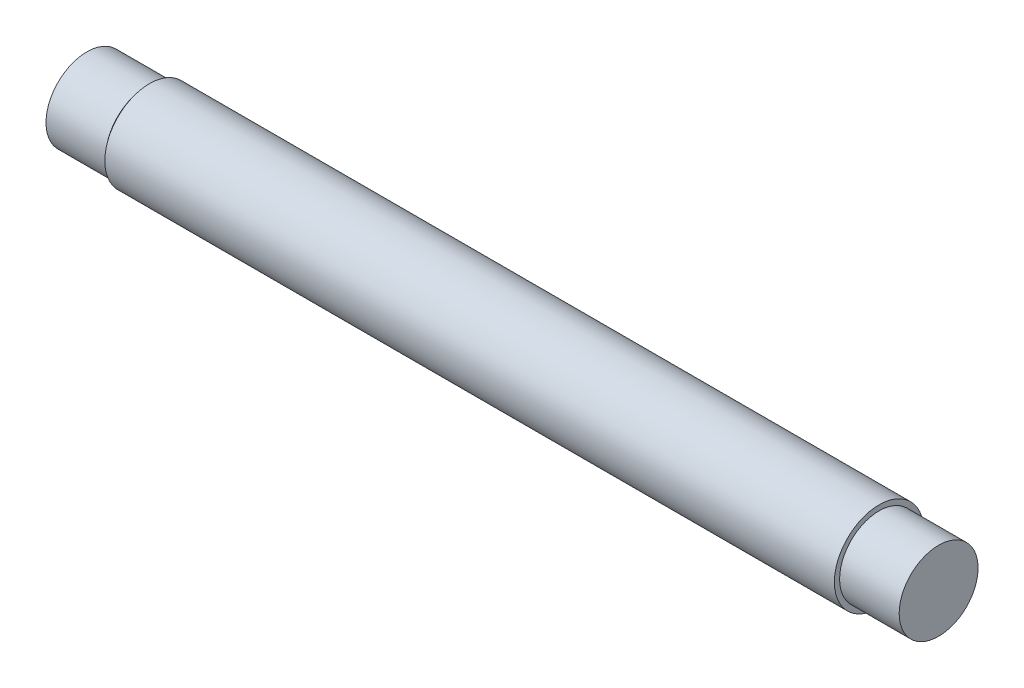
from build123d import *


with BuildPart() as part:
    # 草图1 → 旋转1 (revolve)
    with BuildSketch(Plane.XY, mode=Mode.PRIVATE) as revolve_1_sk:
        Polygon((0, 0), (0, 27.5), (40, 27.5), (40, 26.5), (42, 26.5), (42, 30), (532, 30), (532, 26.5), (572, 26.5), (572, 0), align=None)
    revolve(revolve_1_sk.sketch.rotate(Axis((0, 0, 0), (1, 0, 0)), 90), axis=Axis((0, 0, 0), (1, 0, 0)))


solid = part.part
